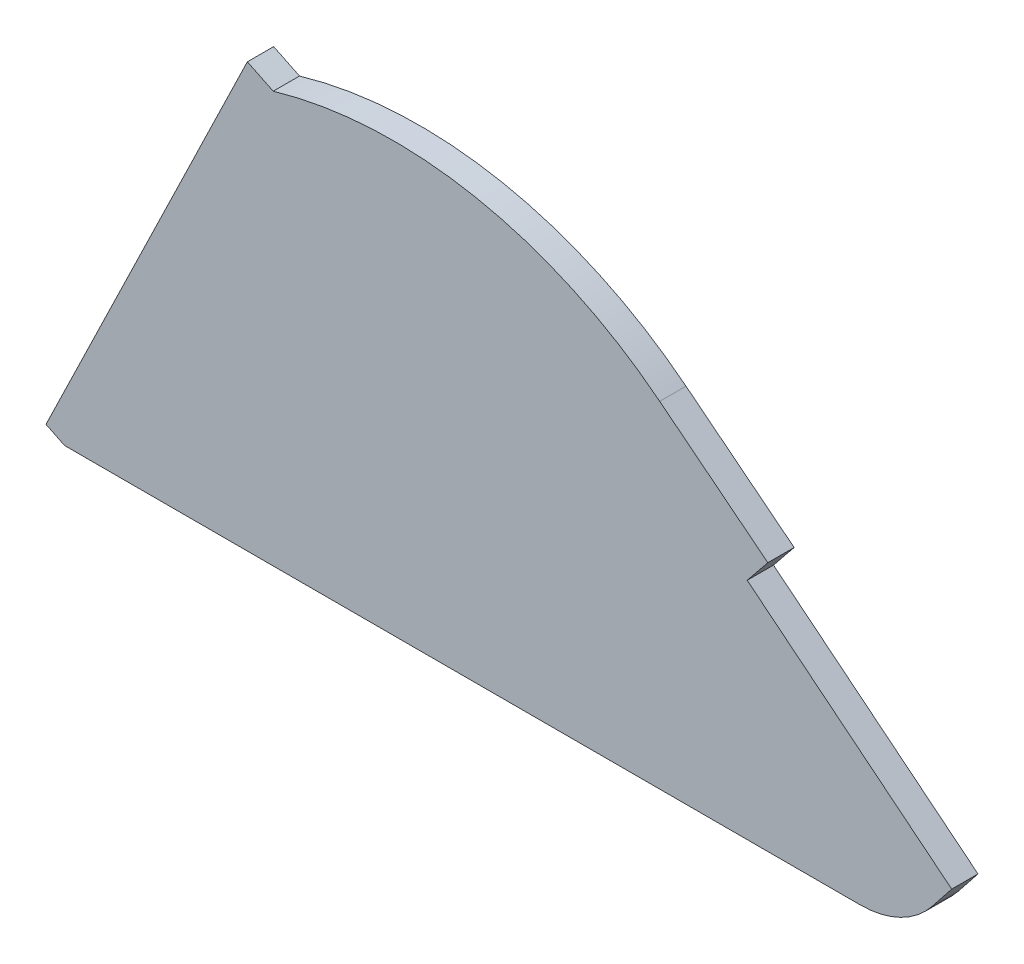
SolidWorks part; units mm, degrees
ref_plane "Front Plane" through (0, 0, 0) normal (0, 0, 1) x (1, 0, 0)
ref_plane "Top Plane" through (0, 0, 0) normal (0, 1, 0) x (1, 0, 0)
ref_plane "Right Plane" through (0, 0, 0) normal (1, 0, 0) x (0, 0, -1)
sketch "Sketch1" plane through (0, 0, 0) normal (0, 0, 1) x (1, 0, 0)
  line L0 (0, 0) -> (605.3417, 0)
  line L1 (139.1, 322.4) -> (-14.1198, 6.8562)
  line L2 (0, 0) -> (-14.1198, 6.8562)
  line L3 (139.1, 322.4) -> (158.7585, 312.8543)
  line L4 (250.4, 103.399) -> (250.4, -89.1712) construction
  line L6 (675, 45.2) -> (519.4, 170.9)
  line L7 (519.4, 170.9) -> (535.1102, 190.3471)
  line L8 (535.1102, 190.3471) -> (452.8433, 255.5244)
  line L9 (675, 45.2) -> (660.2088, 26.5306)
  arc A0 (452.8433, 255.5244) -> (158.7585, 312.8543) centre (250.4, 0) ccw
  arc A1 (605.3417, 0) -> (660.2088, 26.5306) centre (605.3417, 70) ccw
  dimension "D6" = 652
  dimension "D7" = 70
  dimension "D2" = 64.1
  dimension "D3" = 322.4
  dimension "D4" = 139.1
  dimension "D5" = 250.4
  dimension "D8" = 155.6
  dimension "D9" = 170.9
  dimension "D10" = 25
  dimension "D11" = 675
  dimension "D12" = 45.2
extrude "Boss-Extrude1" add sketch "Sketch1" along normal blind 20
